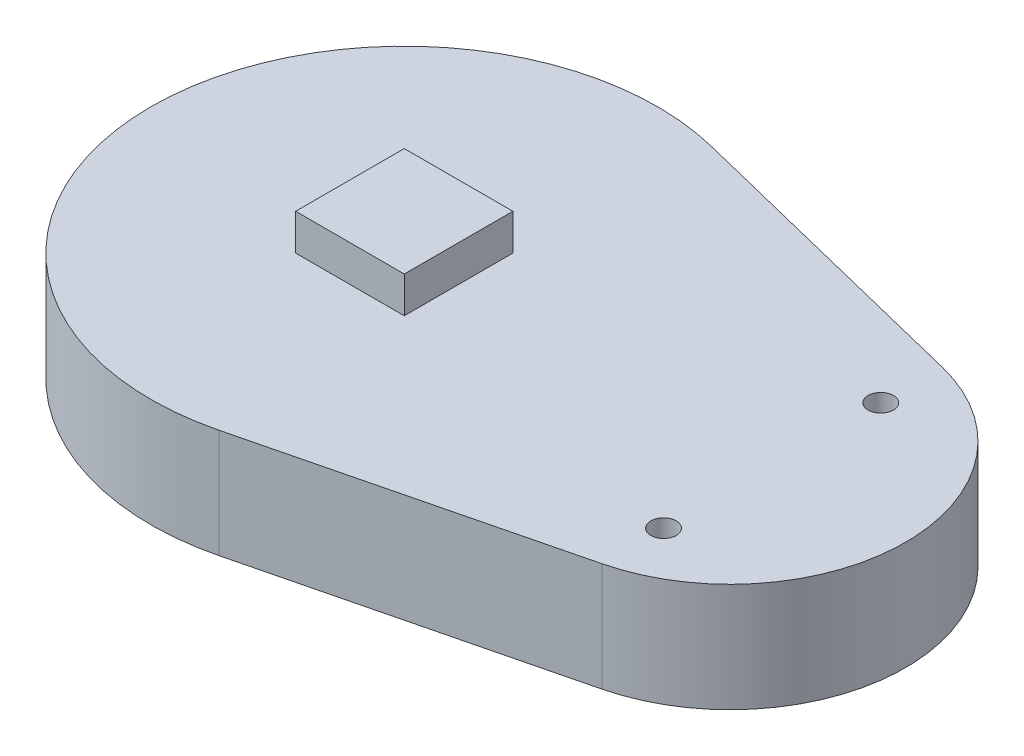
from build123d import *

# Parameters (mm, degrees)
BOSS_EXTRUDE1_DEPTH                      = 30
SKETCH2_W                                = 30
SKETCH2_H                                = 30
BOSS_EXTRUDE2_DEPTH                      = 10
SKETCH3_R                                = 65
BOSS_EXTRUDE3_DEPTH                      = 3.01
SKETCH4_R                                = 30
BOSS_EXTRUDE4_DEPTH                      = 8
CBORE_FOR_M6_PAN_HEAD_SCREW1_D           = 7
CBORE_FOR_M6_PAN_HEAD_SCREW1_DEPTH       = 50.5
CBORE_FOR_M6_PAN_HEAD_SCREW1_CBORE_D     = 13
CBORE_FOR_M6_PAN_HEAD_SCREW1_CBORE_DEPTH = 4.6
CBORE_FOR_M6_PAN_HEAD_SCREW1_TIP         = 2.103012167


with BuildPart() as part:
    # Sketch1 → Boss-Extrude1 (new body)
    with BuildSketch(Plane(origin=(0, 0, 0), x_dir=(1, 0, 0), z_dir=(0, 1, 0))):
        with BuildLine():
            Line((11.612208492, 155.9994544), (-73.209898492, 176.956548554))
            ThreePointArc((-73.209898492, 176.956548554), (-160, 109), (-73.209898492, 41.043451446))
            Line((-73.209898492, 41.043451446), (11.610000013, 61.999999948))
            Line((11.610000013, 61.999999948), (11.612208492, 62.0005456))
            ThreePointArc((11.612208492, 62.0005456), (48.412726633, 109), (11.612208492, 155.9994544))
        make_face()
    extrude(amount=BOSS_EXTRUDE1_DEPTH)

    # Sketch2 → Boss-Extrude2 (add)
    with BuildSketch(Plane(origin=(0, 30, 0), x_dir=(1, 0, 0), z_dir=(0, 1, 0))):
        with Locations((-90, 109)):
            Rectangle(SKETCH2_W, SKETCH2_H)
    extrude(amount=BOSS_EXTRUDE2_DEPTH)

    # Sketch3 → Boss-Extrude3 (add)
    with BuildSketch(Plane.XZ):
        with Locations(Location((-90, -109, 0), (0, 0, 90))):
            Circle(SKETCH3_R)
    extrude(amount=BOSS_EXTRUDE3_DEPTH)

    # Sketch4 → Boss-Extrude4 (add)
    with BuildSketch(Plane.XZ.offset(3.01)):
        with Locations(Location((-90, -109, 0), (0, 0, 270))):
            Circle(SKETCH4_R)
    extrude(amount=BOSS_EXTRUDE4_DEPTH)

    # CBORE for M6 Pan Head Screw1
    with Locations(Plane(origin=(11.612208492, 0, -79), x_dir=(0, 0, -1), z_dir=(0, -1, 0))):
        with Locations((0, 0), (60, 0)):
            CounterBoreHole(CBORE_FOR_M6_PAN_HEAD_SCREW1_D / 2, CBORE_FOR_M6_PAN_HEAD_SCREW1_CBORE_D / 2, CBORE_FOR_M6_PAN_HEAD_SCREW1_CBORE_DEPTH, depth=CBORE_FOR_M6_PAN_HEAD_SCREW1_DEPTH)
            with Locations((0, 0, -(CBORE_FOR_M6_PAN_HEAD_SCREW1_DEPTH + CBORE_FOR_M6_PAN_HEAD_SCREW1_TIP / 2))):  # 118° drill point
                Cone(0, CBORE_FOR_M6_PAN_HEAD_SCREW1_D / 2, CBORE_FOR_M6_PAN_HEAD_SCREW1_TIP, mode=Mode.SUBTRACT)


solid = part.part
